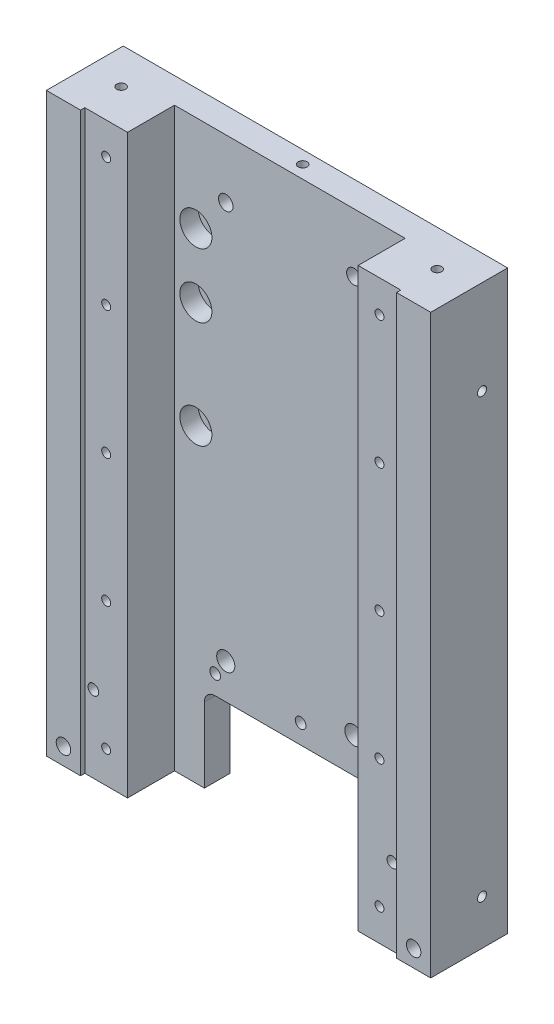
SolidWorks part; units mm, degrees
material "6061Al"
ref_plane "前视基准面" through (0, 0, 0) normal (0, 0, 1) x (1, 0, 0)
ref_plane "上视基准面" through (0, 0, 0) normal (0, 1, 0) x (1, 0, 0)
ref_plane "右视基准面" through (0, 0, 0) normal (1, 0, 0) x (0, 0, -1)
sketch "草图1" plane through (0, 0, 0) normal (0, 0, 1) x (1, 0, 0)
  line L1 (-90, -135) -> (90, -135)
  line L2 (-90, -135) -> (-90, 135)
  line L3 (-90, 135) -> (90, 135)
  line L4 (90, -135) -> (90, 135)
  line L5 (-90, -135) -> (90, 135) construction
  line L6 (-90, 135) -> (90, -135) construction
  point P0 (0, 0)
  dimension "D1" = 180
  dimension "D2" = 270
extrude "凸台-拉伸1" add sketch "草图1" along normal blind 34
sketch "草图2" plane through (0, -135, 0) normal (0, -1, 0) x (1, 0, 0)
  line L0 (0, 34) -> (0, 0) construction
  line L1 (-90, 34) -> (90, 34) construction
  line L2 (-90, 0) -> (90, 0) construction
  line L3 (-54, 34) -> (54, 34)
  line L4 (-54, 34) -> (-54, 12)
  line L5 (-54, 12) -> (54, 12)
  line L6 (54, 34) -> (54, 12)
  dimension "D1" = 12
  dimension "D2" = 108
extrude "切除-拉伸1" cut sketch "草图2" against normal through all
sketch "草图3" plane through (0, 0, 34) normal (0, 0, 1) x (1, 0, 0)
  line L0 (-90, -135) -> (-54, -135) construction
  line L1 (-90, 135) -> (-74, 135)
  line L2 (-90, 135) -> (-90, -135)
  line L3 (-90, -135) -> (-74, -135)
  line L4 (-74, 135) -> (-74, -135)
  line L5 (0, 0) -> (0, -219.5469) construction
  line L6 (-54, 135) -> (-54, -135) construction
  line L7 (74, 135) -> (74, -135)
  line L8 (90, -135) -> (74, -135)
  line L9 (90, 135) -> (90, -135)
  line L10 (90, 135) -> (74, 135)
  dimension "D1" = 20
extrude "凸台-拉伸2" add sketch "草图3" along normal blind 2
hole_wizard "M8 螺纹孔1" positions "草图4" profile "草图5" tap size "M8" standard "ISO"
sketch "草图4" plane through (0, 0, 36) normal (0, 0, 1) x (1, 0, 0)
  line L0 (-82, -135) -> (-82, -114.6979)
  line L1 (-90, -135) -> (-74, -135) construction
  line L2 (0, 0) -> (0, -209.6498) construction
  line L4 (0, 0) -> (124.0498, 0) construction
  line L6 (82, -135) -> (82, -114.6979)
  point P0 (-82, -127)
  point P20 (82, -127)
  dimension "D1" = 8
sketch "草图5" plane through (-82, -127, 36) normal (1, 0, 0) x (0, -1, 0)
  line L0 (0, 0) -> (0, 21.7929)
  line L1 (0, 21.7929) -> (3.4, 19.75)
  line L2 (3.4, 19.75) -> (3.4, 0)
  line L5 (3.4, 0) -> (0, 0)
  line L10 (0, 21.7929) -> (-3.4, 19.75) construction
  line L11 (0, -6.35) -> (0, 107.95) construction
  dimension "螺纹孔钻头直径" = 6.8
  dimension "螺纹孔钻头深度" = 19.75
  dimension "导头角度" = 118
sketch "草图6" plane through (0, 0, 12) normal (0, 0, 1) x (1, 0, 0)
  line L0 (0, 0) -> (0, -135) construction
  line L1 (-54, -135) -> (54, -135) construction
  line L3 (-40, -135) -> (40, -135)
  line L4 (-40, -135) -> (-40, -95)
  line L5 (-40, -95) -> (40, -95)
  line L6 (40, -135) -> (40, -95)
  line L7 (-40, -135) -> (40, -95) construction
  line L8 (-40, -95) -> (40, -135) construction
  point P5 (0, -115)
  dimension "D1" = 80
  dimension "D2" = 40
extrude "切除-拉伸2" cut sketch "草图6" against normal through all
fillet "圆角1" radius 5 2 edges at (40, -95, 6) (-40, -95, 6)
hole_wizard "M5 螺纹孔1" positions "草图7" profile "草图8" tap size "M5" standard "ISO"
sketch "草图7" plane through (0, 135, 0) normal (0, 1, 0) x (1, 0, 0)
  line L0 (0, 0) -> (0, -12)
  line L1 (-54, -12) -> (54, -12) construction
  line L3 (-74, -34) -> (-74, 0)
  line L4 (90, 0) -> (-90, 0) construction
  line L6 (74, -34) -> (74, 0)
  point P0 (-74, -17)
  point P2 (74, -17)
  point P4 (0, -6)
sketch "草图8" plane through (-74, 135, 17) normal (1, 0, 0) x (0, 0, 1)
  line L0 (0, 0) -> (0, 13.6618)
  line L1 (0, 13.6618) -> (2.1, 12.4)
  line L2 (2.1, 12.4) -> (2.1, 0)
  line L5 (2.1, 0) -> (0, 0)
  line L10 (0, 13.6618) -> (-2.1, 12.4) construction
  line L11 (0, -6.35) -> (0, 107.95) construction
  dimension "螺纹孔钻头直径" = 4.2
  dimension "螺纹孔钻头深度" = 12.4
  dimension "导头角度" = 118
cosmetic thread "孔螺蚊线1" parameters "D1"=10, "D2"=5
cosmetic thread "孔螺蚊线2" parameters "D1"=10, "D2"=5
cosmetic thread "孔螺蚊线3" parameters "D1"=10, "D2"=5
hole_wizard "M6 螺纹孔1" positions "草图9" profile "草图10" tap size "M6" standard "ISO"
sketch "草图9" plane through (0, 0, 0) normal (0, 0, -1) x (-1, 0, 0)
  point P0 (-45.0422, -86)
  point P3 (-5.0422, -86)
  point P6 (34.9578, -86)
sketch "草图10" plane through (45.0422, -86, 0) normal (1, 0, 0) x (0, 1, 0)
  line L0 (0, 0) -> (0, 16.5022)
  line L1 (0, 16.5022) -> (2.5, 15)
  line L2 (2.5, 15) -> (2.5, 0)
  line L5 (2.5, 0) -> (0, 0)
  line L10 (0, 16.5022) -> (-2.5, 15) construction
  line L11 (0, -6.35) -> (0, 107.95) construction
  dimension "螺纹孔钻头直径" = 5
  dimension "螺纹孔钻头深度" = 15
  dimension "导头角度" = 118
cosmetic thread "孔螺蚊线6" parameters "D1"=12, "D2"=6
cosmetic thread "孔螺蚊线47" parameters "D1"=12, "D2"=6
cosmetic thread "孔螺蚊线48" parameters "D1"=12, "D2"=6
hole_wizard "M8 螺纹孔2" positions "草图13" profile "草图14" tap size "M8" standard "ISO" end condition through all
sketch "草图13" plane through (0, 0, 12) normal (0, 0, 1) x (1, 0, 0)
  point P0 (-30, 107.5)
  point P3 (30, 107.5)
sketch "草图14" plane through (-30, 107.5, 12) normal (1, 0, 0) x (0, -1, 0)
  line L0 (0, 0) -> (0, 12)
  line L1 (0, 12) -> (3.4, 12)
  line L2 (3.4, 12) -> (3.4, 0)
  line L5 (3.4, 0) -> (0, 0)
  line L11 (0, -6.35) -> (0, 107.95) construction
  dimension "通孔螺纹孔钻头直径" = 6.8
  dimension "通孔螺纹孔钻头深度" = 12
cosmetic thread "孔螺蚊线21" parameters "D2"=8
cosmetic thread "孔螺蚊线22" parameters "D2"=8
hole_wizard "M10 螺纹孔1" positions "草图15" profile "草图16" tap size "M10" standard "ISO" end condition through all
sketch "草图15" plane through (0, 0, 12) normal (0, 0, 1) x (1, 0, 0)
  point P0 (-30, -78.5)
  point P3 (30, -78.5)
sketch "草图16" plane through (-30, -78.5, 12) normal (1, 0, 0) x (0, -1, 0)
  line L0 (0, 0) -> (0, 12)
  line L1 (0, 12) -> (4.25, 12)
  line L2 (4.25, 12) -> (4.25, 0)
  line L5 (4.25, 0) -> (0, 0)
  line L11 (0, -6.35) -> (0, 107.95) construction
  dimension "通孔螺纹孔钻头直径" = 8.5
  dimension "通孔螺纹孔钻头深度" = 12
cosmetic thread "孔螺蚊线23" parameters "D2"=10
cosmetic thread "孔螺蚊线24" parameters "D2"=10
hole_wizard "M8 六角凹头螺钉的柱形沉头孔1" positions "草图17" profile "草图18" counterbore size "M8" standard "ISO" end condition through all
sketch "草图17" plane through (0, 0, 12) normal (0, 0, 1) x (1, 0, 0)
  line L0 (0, 0) -> (0, 182.2274) construction
  line L3 (0, 60) -> (146.4445, 60) construction
  line L5 (-54, 135) -> (54, 135) construction
  point P0 (-44, 90.0389)
  point P6 (-44, 10)
  point P33 (-44, 60)
  point P43 (44, 60)
  point P44 (44, 10)
  point P45 (44, 90.0389)
  dimension "D1" = 75
  dimension "D2" = 88
  dimension "D3" = 30.0389
  dimension "D4" = 50
sketch "草图18" plane through (-44, 90.0389, 12) normal (1, 0, 0) x (0, -1, 0)
  line L0 (0, 0) -> (0, 12)
  line L1 (0, 12) -> (4.5, 12)
  line L3 (4.5, 12) -> (4.5, 8.6)
  line L4 (4.5, 8.6) -> (7.5, 8.6)
  line L5 (7.5, 8.6) -> (7.5, 0)
  line L7 (7.5, 0) -> (0, 0)
  line L11 (0, -6.35) -> (0, 107.95) construction
  dimension "通孔孔直径" = 9
  dimension "通孔孔深度" = 12
  dimension "柱形沉头孔直径" = 15
  dimension "柱形沉头孔深度" = 8.6
hole_wizard "M5 螺纹孔3" positions "草图19" profile "草图20" tap size "M5" standard "ISO"
sketch "草图19" plane through (-90, 0, 0) normal (-1, 0, 0) x (0, 0, 1)
  line L0 (12, 93.9) -> (12, 88.1)
  line L1 (9.5, 93.9) -> (14.5, 93.9) construction
  line L2 (9.5, 88.1) -> (14.5, 88.1) construction
  line L4 (12, -111.1) -> (12, -116.9)
  line L5 (9.5, -111.1) -> (14.5, -111.1) construction
  line L6 (9.5, -116.9) -> (14.5, -116.9) construction
  point P0 (12, 91)
  point P2 (12, -114)
sketch "草图20" plane through (-90, 91, 12) normal (0, 1, 0) x (0, 0, 1)
  line L0 (0, 0) -> (0, 13.6618)
  line L1 (0, 13.6618) -> (2.1, 12.4)
  line L2 (2.1, 12.4) -> (2.1, 0)
  line L5 (2.1, 0) -> (0, 0)
  line L10 (0, 13.6618) -> (-2.1, 12.4) construction
  line L11 (0, -6.35) -> (0, 107.95) construction
  dimension "螺纹孔钻头直径" = 4.2
  dimension "螺纹孔钻头深度" = 12.4
  dimension "导头角度" = 118
cosmetic thread "孔螺蚊线25" parameters "D1"=10, "D2"=5
cosmetic thread "孔螺蚊线26" parameters "D1"=10, "D2"=5
hole_wizard "M5 螺纹孔4" positions "草图21" profile "草图22" tap size "M5" standard "ISO"
sketch "草图21" plane through (90, 0, 0) normal (1, 0, 0) x (0, 0, -1)
  point P0 (-12, 91)
  point P3 (-12, -114)
sketch "草图22" plane through (90, 91, 12) normal (0, 1, 0) x (0, 0, -1)
  line L0 (0, 0) -> (0, 13.6618)
  line L1 (0, 13.6618) -> (2.1, 12.4)
  line L2 (2.1, 12.4) -> (2.1, 0)
  line L5 (2.1, 0) -> (0, 0)
  line L10 (0, 13.6618) -> (-2.1, 12.4) construction
  line L11 (0, -6.35) -> (0, 107.95) construction
  dimension "螺纹孔钻头直径" = 4.2
  dimension "螺纹孔钻头深度" = 12.4
  dimension "导头角度" = 118
cosmetic thread "孔螺蚊线27" parameters "D1"=10, "D2"=5
cosmetic thread "孔螺蚊线28" parameters "D1"=10, "D2"=5
hole_wizard "M6 螺纹孔2" positions "草图23" profile "草图24" tap size "M6" standard "ISO" end condition through all
sketch "草图23" plane through (0, 0, 0) normal (0, 0, -1) x (-1, 0, 0)
  line L0 (-40, -135) -> (-90, -135) construction
  line L1 (-90, -135) -> (-90, 135) construction
  line L2 (0, 0) -> (0, -163.5434) construction
  point P0 (-70, -99)
  point P12 (70, -99)
  dimension "D1" = 36
  dimension "D2" = 20
sketch "草图24" plane through (70, -99, 0) normal (1, 0, 0) x (0, 1, 0)
  line L0 (0, 0) -> (0, 36)
  line L1 (0, 36) -> (2.5, 36)
  line L2 (2.5, 36) -> (2.5, 0)
  line L5 (2.5, 0) -> (0, 0)
  line L11 (0, -6.35) -> (0, 107.95) construction
  dimension "通孔螺纹孔钻头直径" = 5
  dimension "通孔螺纹孔钻头深度" = 36
cosmetic thread "孔螺蚊线29" parameters "D2"=6
cosmetic thread "孔螺蚊线30" parameters "D2"=6
hole_wizard "M4 螺纹孔1" positions "草图25" profile "草图26" tap size "M4" standard "ISO"
sketch "草图25" plane through (0, 0, 0) normal (0, 0, -1) x (-1, 0, 0)
  line L0 (-90, -135) -> (-90, 135) construction
  line L1 (-40, -135) -> (-90, -135) construction
  line L2 (0, 0) -> (0, -194.1978) construction
  point P0 (-87, 32)
  point P3 (-87, -47)
  point P6 (-87, -126)
  point P23 (87, -126)
  point P24 (87, -47)
  point P25 (87, 32)
  dimension "D1" = 3
  dimension "D2" = 9
  dimension "D3" = 79
  dimension "D4" = 79
sketch "草图26" plane through (87, 32, 0) normal (1, 0, 0) x (0, 1, 0)
  line L0 (0, 0) -> (0, 11.0914)
  line L1 (0, 11.0914) -> (1.65, 10.1)
  line L2 (1.65, 10.1) -> (1.65, 0)
  line L5 (1.65, 0) -> (0, 0)
  line L10 (0, 11.0914) -> (-1.65, 10.1) construction
  line L11 (0, -6.35) -> (0, 107.95) construction
  dimension "螺纹孔钻头直径" = 3.3
  dimension "螺纹孔钻头深度" = 10.1
  dimension "导头角度" = 118
cosmetic thread "孔螺蚊线31" parameters "D1"=8, "D2"=4
cosmetic thread "孔螺蚊线32" parameters "D1"=8, "D2"=4
cosmetic thread "孔螺蚊线33" parameters "D1"=8, "D2"=4
cosmetic thread "孔螺蚊线34" parameters "D1"=8, "D2"=4
cosmetic thread "孔螺蚊线35" parameters "D1"=8, "D2"=4
cosmetic thread "孔螺蚊线36" parameters "D1"=8, "D2"=4
hole_wizard "M5 螺纹孔5" positions "草图27" profile "草图28" tap size "M5" standard "ISO"
sketch "草图27" plane through (0, 0, 34) normal (0, 0, 1) x (1, 0, 0)
  line L0 (-64, 135) -> (-64, -135) construction
  line L1 (-54, 135) -> (-74, 135) construction
  line L2 (-74, -135) -> (-54, -135) construction
  line L4 (0, 0) -> (122.6008, 0) construction
  line L6 (0, 0) -> (0, 176.4948) construction
  line L8 (-64, 0) -> (-64, 60) construction
  line L9 (64, 0) -> (64, 60) construction
  point P0 (-64, 0)
  point P23 (-64, 60)
  point P24 (-64, 120)
  point P27 (-64, -120)
  point P28 (-64, -60)
  point P31 (64, -60)
  point P32 (64, -120)
  point P33 (64, 120)
  point P34 (64, 60)
  point P35 (64, 0)
  dimension "D1" = 3
  dimension "D2" = 60
sketch "草图28" plane through (-64, 0, 34) normal (1, 0, 0) x (0, -1, 0)
  line L0 (0, 0) -> (0, 13.6618)
  line L1 (0, 13.6618) -> (2.1, 12.4)
  line L2 (2.1, 12.4) -> (2.1, 0)
  line L5 (2.1, 0) -> (0, 0)
  line L10 (0, 13.6618) -> (-2.1, 12.4) construction
  line L11 (0, -6.35) -> (0, 107.95) construction
  dimension "螺纹孔钻头直径" = 4.2
  dimension "螺纹孔钻头深度" = 12.4
  dimension "导头角度" = 118
cosmetic thread "孔螺蚊线37" parameters "D1"=10, "D2"=5
cosmetic thread "孔螺蚊线38" parameters "D1"=10, "D2"=5
cosmetic thread "孔螺蚊线39" parameters "D1"=10, "D2"=5
cosmetic thread "孔螺蚊线40" parameters "D1"=10, "D2"=5
cosmetic thread "孔螺蚊线41" parameters "D1"=10, "D2"=5
cosmetic thread "孔螺蚊线42" parameters "D1"=10, "D2"=5
cosmetic thread "孔螺蚊线43" parameters "D1"=10, "D2"=5
cosmetic thread "孔螺蚊线44" parameters "D1"=10, "D2"=5
cosmetic thread "孔螺蚊线45" parameters "D1"=10, "D2"=5
cosmetic thread "孔螺蚊线46" parameters "D1"=10, "D2"=5
